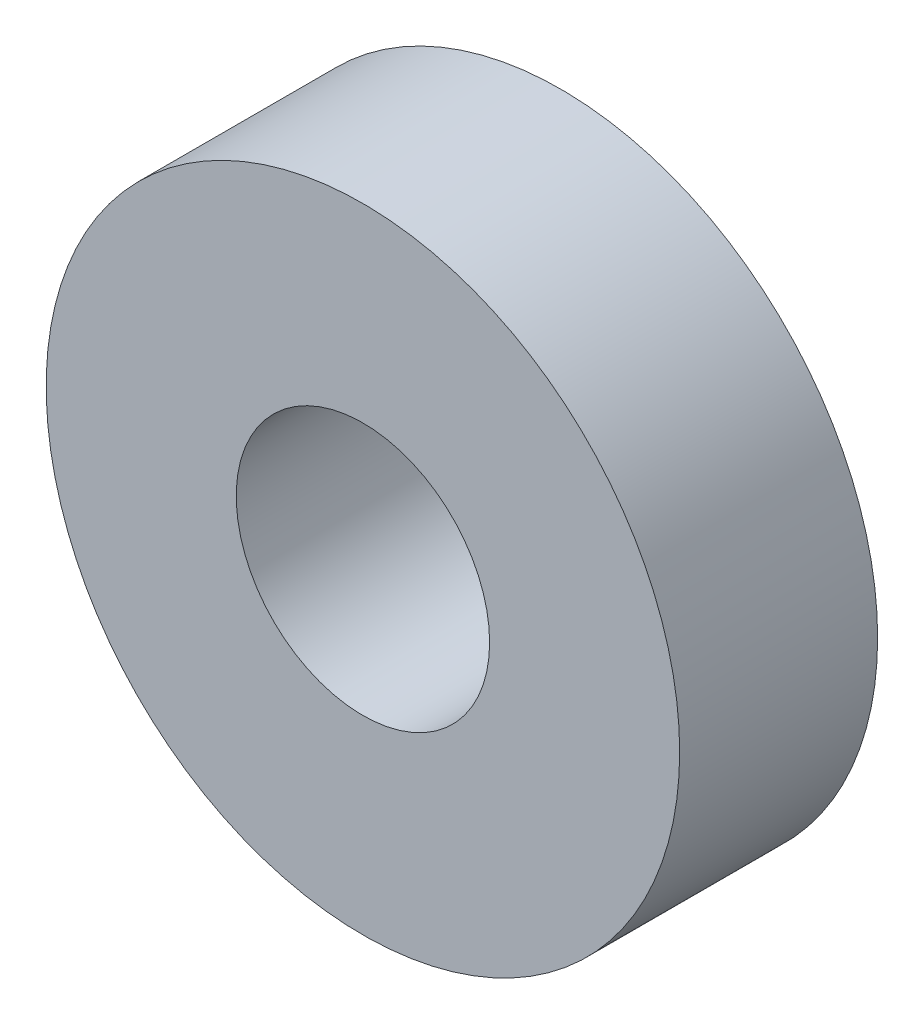
from build123d import *

# Parameters (mm, degrees)
SKETCH_1_R      = 8
SKETCH_1_R_2    = 3.2
EXTRUDE_1_DEPTH = 2.5


with BuildPart() as part:
    # 草图1 → 凸台-拉伸1 (new, symmetric)
    with BuildSketch(Plane.XY):
        Circle(SKETCH_1_R)
        Circle(SKETCH_1_R_2, mode=Mode.SUBTRACT)
    extrude(amount=EXTRUDE_1_DEPTH, both=True)


solid = part.part
